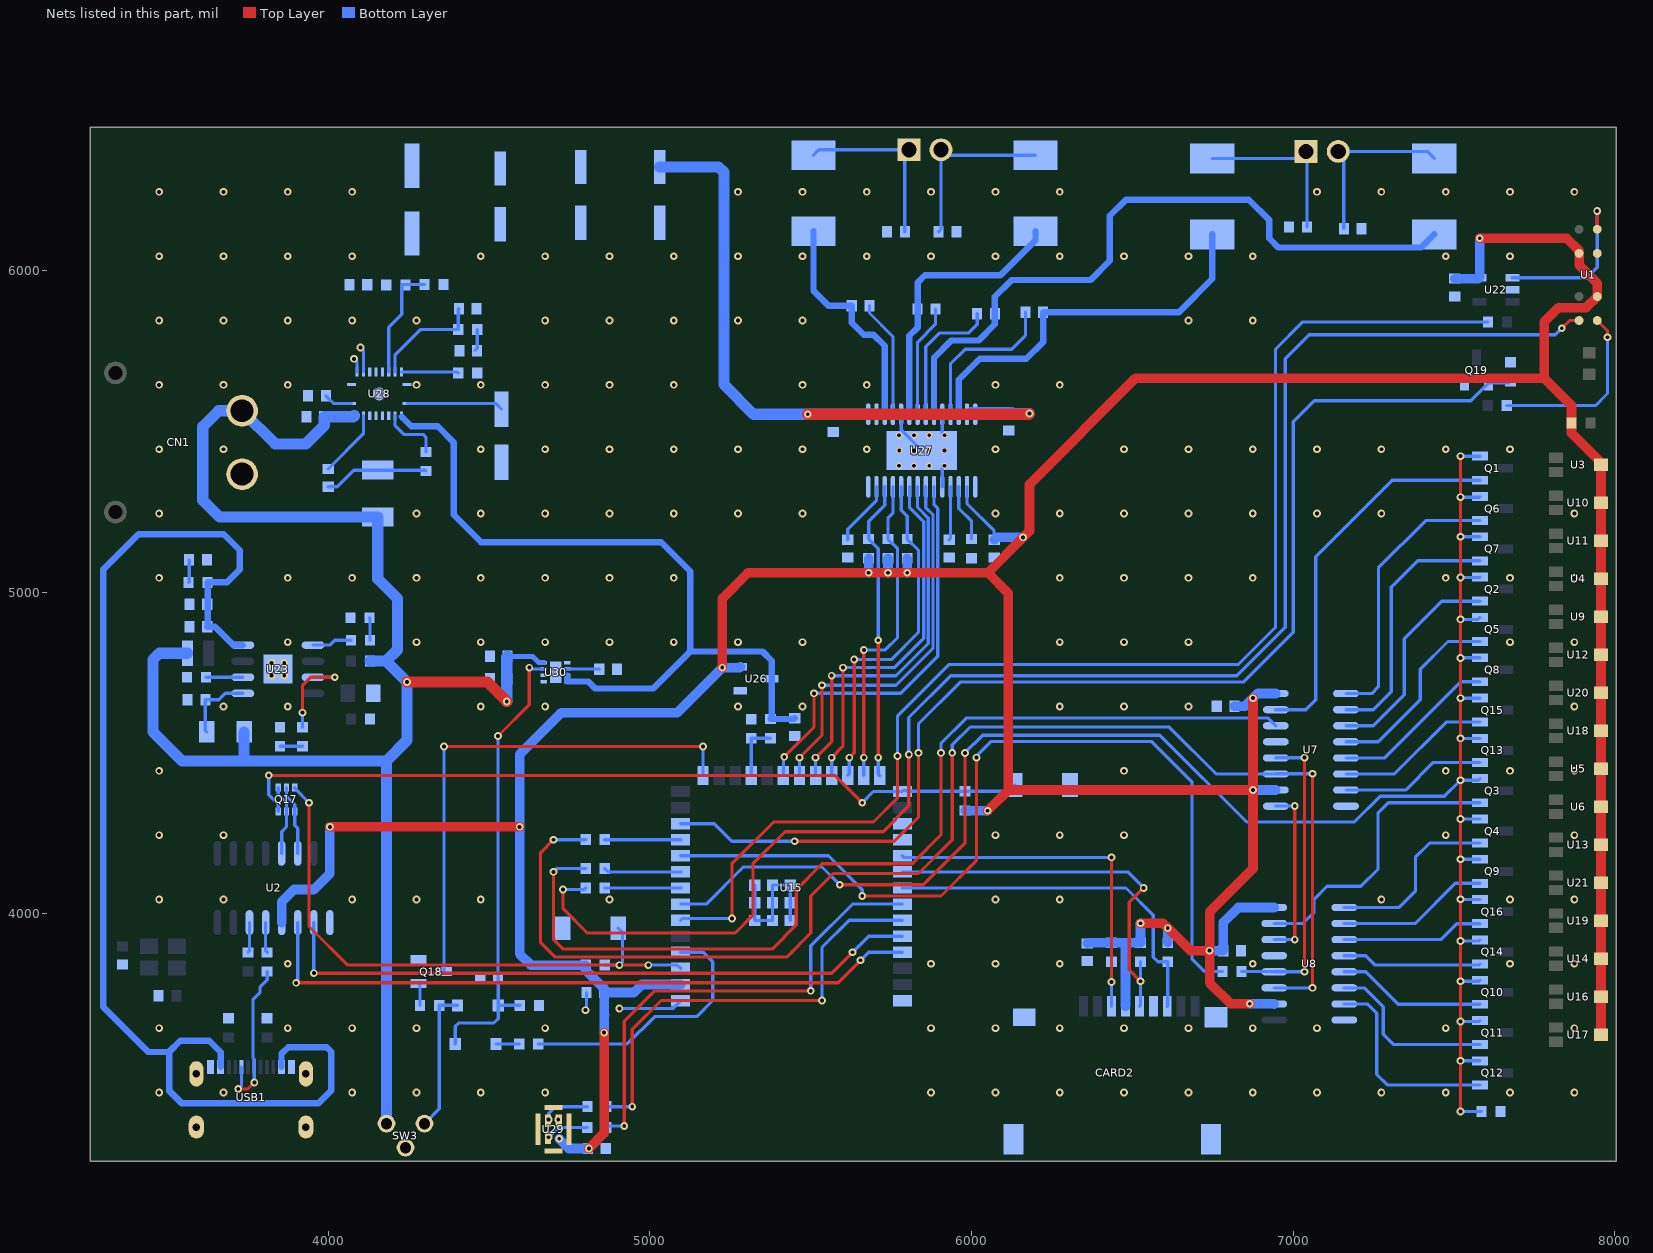
[diagram p0: the nets of this part, all layers, seen from the top]
# Altium PCB MISC75432.pcbdoc (part 2 of 2)
Units mil, origin at the board's own origin, x right, y up, seen from the top; angles counter-clockwise.
Board outline 4745 x 3215 mil, 2 copper layers (Top Layer, Bottom Layer), stack 62.206 mil thick; 150 components, 141 nets, 533 pads, 333 vias.

## Via types
v1: diameter 24.02, hole 12, Top Layer to Bottom Layer, 317 vias
v2: diameter 19.69, hole 11.8, Top Layer to Bottom Layer, 12 vias
v3: diameter 24, hole 12, Top Layer to Bottom Layer, 4 vias

## Nets (pads, with @x,y where several pads share a name; then routed paths per layer and width w, separated by ;. In a path a pad name is that pad's centre, name@x,y a point inside that pad or via, vN(x,y) a via of type N, cw(c..) or ccw(c..) an arc to the next point about the centre after c; other vN are vias at no path point) (continued)
$2N126: R16.1 U23.6 | length 114.7
  Bottom Layer w10: R16.1@3619.66,4735 U23.6@3734.37,4735
$2N139: C10.1 R19.2 | length 70.9
  Bottom Layer w10: R19.2@3565.34,5030 3567.44,5032.1 C10.1@3567.44,5100
$2N141: C9.2 R20.1 U23.5 | length 226.7
  Bottom Layer w10: R20.1@3621.78,4565 3617.68,4569.1 C9.2@3617.68,4665 3660,4665 3680,4685 U23.5@3734.37,4685
$2N142: LED2.2 R21.1 | length 70.1
  Bottom Layer w10: LED2.2@3849.99,4520.51 3919.83,4520.51 R21.1@3920,4520.34
$2N143: R21.2 U23.3 | length 308
  Top Layer w10: v1(3920,4625) 3920,4710 3945,4735 v1(4020,4735)
  Bottom Layer w10: R21.2@3920,4579.66 v1(3920,4625) ; U23.3@3952.67,4735 v1(4020,4735)
$2N144: R17.2 U23.1 | length 123.9
  Bottom Layer w10: U23.1@3952.67,4835 4005,4835 4020,4850 R17.2@4070.34,4850
$2N145: LED1.2 R17.1 | length 70.5
  Bottom Layer w10: LED1.2@4128.46,4919.98 4129.66,4918.79 R17.1@4129.66,4850
$2N168: D2.1 R26.2 | length 71.9
  Bottom Layer w10: D2.1@4521.57,3595.01 R26.2@4593.52,3595.01
$2N172: Q18.1 R27.1 | length 69.6
  Bottom Layer w10: Q18.1@4280.63,3782.6 4285.34,3777.89 R27.1@4285.34,3715
$2N183: C17.2 U28.1 | length 301.3
  Bottom Layer w10: U28.1@4244.44,5586.46 4520.62,5586.46 C17.2@4538.41,5568.66
$2N185: C18.2 L1.1 R30.2 U28.4 U28.5 U28.6 U28.7 | length 325.7
  Bottom Layer w10: C18.2@4000,5327.44 4027.32,5327.44 4078.69,5378.82 L1.1@4153.41,5378.82 4300.92,5378.82 R30.2@4303.41,5376.33
$2N186: R30.1 U28.3 | length 187.2
  Bottom Layer w10: U28.3@4207.55,5547.99 4207.55,5517.45 4235,5490 4295,5490 4303.41,5481.59 R30.1@4303.41,5435.65
$2N187: C18.1 U28.8 | length 210.6
  Bottom Layer w10: C18.1@4000,5382.56 4109.12,5491.68 U28.8@4109.12,5547.99
$2N197: R33.2 U28.19 | length 177.8
  Bottom Layer w10: U28.19@4227.23,5683.99 4400.75,5683.99 R33.2@4403.75,5680.99
$2N200: C20.1 R34.2 | length 68
  Bottom Layer w10: C20.1@4455.85,5750.99 4463.07,5758.21 R34.2@4463.07,5815.99
$2N209: R35.2 U27.3 | length 179
  Bottom Layer w10: U27.3@5960.16,5327.18 5960.16,5259.84 6000,5220 R35.2@6000,5164.66
$2N210: C27.1 U27.4 | length 166.5
  Bottom Layer w10: C27.1@5930,5162.56 5934.57,5167.13 U27.4@5934.57,5327.18
$2N219: C28.2 U27.13 | length 201.6
  Bottom Layer w10: C28.2@5615,5162.56 5615,5195 5704.25,5284.25 U27.13@5704.25,5327.18
$2N224: C33.1 U27.18 | length 367.4
  Bottom Layer w10: C33.1@5682.56,5890 5682.56,5867.44 5755.43,5794.57 U27.18@5755.43,5552.82
$2N227: C34.1 U27.21 | length 350.1
  Bottom Layer w10: U27.21@5832.2,5552.82 5832.2,5777.2 5887.56,5832.56 C34.1@5887.56,5880
$2N228: C35.1 U27.22 | length 431
  Bottom Layer w10: U27.22@5857.79,5552.82 5857.79,5762.79 5900,5805 5990,5805 6017.44,5832.44 C35.1@6017.44,5865
$2N231: C36.1 U27.25 | length 498.6
  Bottom Layer w10: U27.25@5934.57,5552.82 5934.57,5709.57 5980,5755 6125,5755 6167.44,5797.44 C36.1@6167.44,5870
$2N241: U15.29
$2N242: U15.30
$2N254: C38.1 CN3.1 L4.2 | length 563.5
  Bottom Layer w10: L4.2@5508.6,6358.11 5525.49,6375 CN3.1@5805,6374.99 5792.56,6362.56 C38.1@5792.56,6120
$2N255: C39.2 CN3.2 L5.2 | length 558.7
  Bottom Layer w10: C39.2@5897.44,6120 5905,6127.56 CN3.2@5905,6374.99 5921.89,6358.11 L5.2@6198.6,6358.11
$2N256: C30.1 CN2.1 L2.2 | length 536.5
  Bottom Layer w10: L2.2@6748.6,6348.11 7018.11,6348.11 CN2.1@7040,6369.99 7042.56,6367.44 C30.1@7042.56,6135
$2N257: C37.2 CN2.2 L3.2 | length 554.9
  Bottom Layer w10: C37.2@7157.44,6130 7157.44,6352.56 CN2.2@7140,6369.99 7416.71,6370 L3.2@7438.6,6348.11
$2N275: R39.2 U29.3 | length 149.3
  Bottom Layer w10: v1(4685,3360) 4685,3380 4705,3400 R39.2@4806.02,3400
$2N276: R40.2 U29.4 | length 132.6
  Bottom Layer w10: v1(4685,3305) 4715.34,3335.34 R40.2@4805,3335.34
$2N296: R11.2 U15.8 | length 235.9
  Bottom Layer w10: R11.2@4859.66,4080 5095.31,4080 U15.8@5095.51,4079.8
$2N298: R8.1 U15.9 | length 240.1
  Bottom Layer w10: R8.1@4859.66,4140 4869.85,4129.81 U15.9@5095.51,4129.81
$2N300: R9.1 U15.10 | length 2755.8
  Top Layer w10: v1(5660,4055) 5905,4055 6015,4165 v1(6015,4485)
  Bottom Layer w10: U15.10@5095.51,4179.81 5555.19,4179.81 5660,4075 v1(5660,4055) ; v1(6015,4485) 6015,4490 6060,4535 6560,4535 6685,4410 6685,3860 6725,3820 R9.1@6780.34,3820
$2N303: R10.2 U15.11 | length 235.9
  Bottom Layer w10: R10.2@4859.66,4230 4859.85,4229.81 U15.11@5095.51,4229.81
$2N304: D1.1 R27.2 SW3.2 | length 443.4
  Bottom Layer w10: SW3.2@4299.05,3347.4 4344.66,3393.01 R27.2@4344.66,3715 D1.1@4401.61,3715
$2N306: C22.1 U28.10 | length 89.6
  Bottom Layer w10: C22.1@3992.56,5610 4016.1,5586.46 U28.10@4072.39,5586.46
+12V: C19.1 C23.1 C24.1 C25.1 C29.1 C31.2 C32.2 R32.2 U27.15 U27.16 U27.27 U27.28 U28.14 U28.15 U28.16 | length 2234
  Top Layer w35: v1(5490.71,5552.56) 6177.56,5552.56 v1(6180,5555)
  Bottom Layer w35: C25.1@5030,6321.61 5213.39,6321.61 5230,6305 5230,5645 5322.44,5552.56 v1(5490.71,5552.56) C32.2@5570,5552.56 5694.24,5552.56 5694.51,5552.82 ; 5995.49,5552.82 6000.23,5557.56 C31.2@6115,5557.56 ; C31.2@6127.56,5555 v1(6180,5555)
AGND: C1.2 C2.2 C3.2 C4.1 C5.1 C6.2 C7.2 C8.1 C9.1 C10.2 C11.1 C12.2 C13.1 C14.1 C15.2 C16.2 C17.1 C19.2 C20.2 C21.2 C22.2 C23.2 C24.2 C25.2 C26.2 C27.2 C28.1 C29.2 C30.2 C31.1 C32.1 C37.1 C38.2 C39.1 C40.2 C41.2 CARD2.6 CARD2.10 CARD2.11 CARD2.12 CARD2.13 CN1.1 LED1.1 LED2.1 Q18.2 Q19.2 R1.2 R4.1 R7.1 R15.1 R16.2 R18.1 R25.2 R29.1 R31.1 R33.1 R35.1 R42.2 SW1.1 SW2.2 SW3.3 U1.3 U2.1 U7.8 U7.13 U8.8 U8.13 U15.1 U15.40 U15.41 U22.2 U23.9 U26.1 U27.1 U27.5 U27.14 U27.19 U27.24 U27.29 U28.11 U28.12 U28.13 U28.20 U28.21 U29.2 U29.5 U29.6 U29.7 U29.8 U30.5 U30.9 USB1.1 USB1.12 USB1.13 USB1.14 | length 1098.7
  Bottom Layer w10: v1(4080,5725) 4089.44,5715.56 U28.12@4089.44,5683.99 ; v1(4100,5760) 4109.12,5750.88 U28.13@4109.12,5683.99 ; v1(4800,3700) 4802.44,3702.44 C13.1@4802.44,3755 ; v1(4905,3705) 5070.7,3705 U15.1@5095.51,3729.8 ; U15.41@5325.82,4088.86 U15.41@5325.82,4033.74 U15.41@5325.82,3978.62 U15.41@5380.94,3978.62 U15.41@5380.94,4033.74 U15.41@5380.94,4088.86 U15.41@5436.06,4088.86 U15.41@5436.06,4033.74 U15.41@5436.06,3978.62 ; U27.19@5781.02,5552.82 5781.02,5503.98 U27.29@5845,5439.99 ; U27.5@5908.98,5327.18 5908.98,5385.86 v2(5915.87,5392.76) ; U27.24@5908.98,5552.82 5908.98,5494.14 v2(5915.87,5487.24)
  other v1: 4715,3360 3474.1,3444.1 3674.1,3444.1 4074.1,3444.1 4274.1,3444.1 4474.1,3444.1 4674.1,3444.1 5874.1,3444.1 6074.1,3444.1 6274.1,3444.1 6474.1,3444.1 6674.1,3444.1 6874.1,3444.1 7074.1,3444.1 7274.1,3444.1 7474.1,3444.1 7674.1,3444.1 7874.1,3444.1 3474.1,3644.1 3874.1,3644.1 4074.1,3644.1 4274.1,3644.1 4674.1,3644.1 5874.1,3644.1 6074.1,3644.1 6274.1,3644.1 6474.1,3644.1 6674.1,3644.1 6874.1,3644.1 7074.1,3644.1 7474.1,3644.1 7874.1,3644.1 3874.1,3844.1 5874.1,3844.1 6074.1,3844.1 6274.1,3844.1 6874.1,3844.1 7674.1,3844.1 7874.1,3844.1 3474.1,4044.1 3674.1,4044.1 4074.1,4044.1 4274.1,4044.1 4474.1,4044.1 4874.1,4044.1 6074.1,4044.1 6274.1,4044.1 7274.1,4044.1 7674.1,4044.1 7874.1,4044.1 3474.1,4244.1 3674.1,4244.1 6074.1,4244.1 6274.1,4244.1 6474.1,4244.1 7474.1,4244.1 7874.1,4244.1 3474.1,4444.1 6474.1,4444.1 7474.1,4444.1 7674.1,4444.1 7874.1,4444.1 3674.1,4644.1 3874.1,4644.1 4474.1,4644.1 4674.1,4644.1 5274.1,4644.1 5474.1,4644.1 6274.1,4644.1 6474.1,4644.1 6674.1,4644.1 7874.1,4644.1 3874.1,4844.1 4274.1,4844.1 4474.1,4844.1 4674.1,4844.1 4874.1,4844.1 5074.1,4844.1 5274.1,4844.1 5474.1,4844.1 6274.1,4844.1 6474.1,4844.1 6674.1,4844.1 7674.1,4844.1 7874.1,4844.1 3474.1,5044.1 3874.1,5044.1 4074.1,5044.1 4274.1,5044.1 4474.1,5044.1 4674.1,5044.1 4874.1,5044.1 5074.1,5044.1 6274.1,5044.1 6474.1,5044.1 6674.1,5044.1 6874.1,5044.1 7474.1,5044.1 7674.1,5044.1 7874.1,5044.1 3474.1,5244.1 4274.1,5244.1 4474.1,5244.1 4674.1,5244.1 4874.1,5244.1 5074.1,5244.1 5274.1,5244.1 5474.1,5244.1 6074.1,5244.1 6274.1,5244.1 6474.1,5244.1 6674.1,5244.1 6874.1,5244.1 7074.1,5244.1 7274.1,5244.1 7874.1,5244.1 3474.1,5444.1 3674.1,5444.1 4474.1,5444.1 4674.1,5444.1 4874.1,5444.1 5074.1,5444.1 5274.1,5444.1 5474.1,5444.1 5674.1,5444.1 6074.1,5444.1 6474.1,5444.1 6674.1,5444.1 6874.1,5444.1 7074.1,5444.1 7274.1,5444.1 7474.1,5444.1 7674.1,5444.1 3474.1,5644.1 3674.1,5644.1 3874.1,5644.1 4274.1,5644.1 4474.1,5644.1 4674.1,5644.1 4874.1,5644.1 5074.1,5644.1 5474.1,5644.1 5674.1,5644.1 6074.1,5644.1 6274.1,5644.1 3474.1,5844.1 3674.1,5844.1 3874.1,5844.1 4074.1,5844.1 4274.1,5844.1 4674.1,5844.1 4874.1,5844.1 5074.1,5844.1 5274.1,5844.1 5474.1,5844.1 6674.1,5844.1 6874.1,5844.1 3474.1,6044.1 3674.1,6044.1 3874.1,6044.1 4074.1,6044.1 4474.1,6044.1 4674.1,6044.1 4874.1,6044.1 5074.1,6044.1 5274.1,6044.1 5474.1,6044.1 5674.1,6044.1 5874.1,6044.1 6074.1,6044.1 6274.1,6044.1 6474.1,6044.1 6674.1,6044.1 6874.1,6044.1 7474.1,6044.1 7674.1,6044.1 3474.1,6244.1 3674.1,6244.1 3874.1,6244.1 4074.1,6244.1 5274.1,6244.1 5474.1,6244.1 5674.1,6244.1 5874.1,6244.1 6074.1,6244.1 6274.1,6244.1 7074.1,6244.1 7274.1,6244.1 7474.1,6244.1 7674.1,6244.1 7874.1,6244.1
  other v2: 5774.13,5392.76 5821.38,5392.76 5868.62,5392.76 5775,5439.99 5821.38,5439.99 5868.62,5439.99 5915.87,5439.99 5774.13,5487.24 5821.38,5487.24 5868.62,5487.24
  other v3: 3823.84,4740.31 3863.21,4740.31 3823.84,4779.68 3863.21,4779.68
AMP_PDN: R36.2 U15.26 U27.12 | length 933.3
  Top Layer w10: v1(5710,4485) v1(5710,4850)
  Bottom Layer w10: v1(5710,4485) 5710,4434.02 U15.26@5715,4429.02 ; v1(5710,4850) 5710,5134.66 R36.2@5680,5164.66 5680,5220 5729.84,5269.84 U27.12@5729.84,5327.18
AMP_SCL: R38.2 U15.25 U27.11 | length 998.2
  Top Layer w10: v1(5665,4485) v1(5665,4820)
  Bottom Layer w10: U15.25@5665,4430.19 v1(5665,4485) ; v1(5665,4820) 5731.42,4820 5770,4858.58 5770,5134.66 R38.2@5740,5164.66 5740,5230 5755.43,5245.43 U27.11@5755.43,5327.18
AMP_SDA: R37.2 U15.24 U27.10 | length 1077.8
  Top Layer w10: v1(5620,4485) 5635,4500 v1(5635,4790)
  Bottom Layer w10: U15.24@5615,4430.19 5620,4435.19 v1(5620,4485) ; v1(5635,4790) 5750,4790 5835,4875 5835,5129.66 R37.2@5800,5164.66 5800,5235 5781.02,5253.98 U27.10@5781.02,5327.18
BAT_MONITOR: R28.1 R29.2 U15.18 | length 174.9
  Bottom Layer w10: U15.18@5315,4430.19 R29.2@5315,4545.34 5374.32,4545.34 R28.1@5374.66,4545.68
CH340G_RXD: U2.3 U15.37 | length 2113.1
  Top Layer w10: v1(3900,3785) 5585,3785 v1(5655,3855)
  Bottom Layer w10: v1(3900,3785) 3905,3790 U2.3@3905,3972.3 ; v1(5655,3855) 5679.81,3879.8 U15.37@5784.49,3879.8
CH340G_TXD: U2.2 U15.36 | length 2034.3
  Top Layer w10: v1(3955,3815) 5565,3815 v1(5630,3880)
  Bottom Layer w10: v1(3955,3815) U2.2@3955,3972.3 ; v1(5630,3880) 5679.81,3929.8 U15.36@5784.49,3929.8
COMP: C21.1 R34.1 U28.18 | length 348.1
  Bottom Layer w10: U28.18@4207.55,5683.99 4207.55,5737.55 4285.99,5815.99 R34.1@4403.75,5815.99 4403.75,5878.89 C21.1@4405.85,5880.99
CT: C41.1 U30.6 | length 99.8
  Bottom Layer w10: U30.6@4743.1,4761.05 4841.39,4761.05 C41.1@4842.44,4760
D+: R6.1 U2.5 | length 94.7
  Bottom Layer w10: U2.5@3805,3972.3 3805,3884.66 R6.1@3810,3879.66
D-: R5.1 U2.6 | length 94.7
  Bottom Layer w10: R5.1@3750,3879.66 3755,3884.66 U2.6@3755,3972.3
DP1: R6.2 USB1.6 USB1.8 | length 496.4
  Top Layer w10: v1(3720,3455) 3750,3455 v1(3770,3475)
  Bottom Layer w10: v1(3720,3455) 3730,3465 3730,3523.03 USB1.8@3730.47,3523.51 ; v1(3770,3475) 3769.84,3475.16 USB1.6@3769.84,3523.51 3769.84,3546.91 3766,3550.75 3766,3733.84 3788,3755.84 3788,3772.46 3810,3794.46 R6.2@3810,3820.34
DTR: Q17.2 Q17.4 U2.13 | length 221.5
  Bottom Layer w10: Q17.4@3844.41,4392.4 3844.41,4370.59 3870,4345 Q17.2@3870,4317.6 3870,4270 3855,4255 U2.13@3855,4187.7
FB: R31.2 R32.1 U28.17 | length 359.3
  Bottom Layer w10: U28.17@4187.86,5683.99 4187.86,5822.86 4228.07,5863.07 4228.07,5955.99 R31.2@4298.75,5955.99
I2S_LRCK: U15.20 U27.6 | length 1258.8
  Top Layer w10: v1(5417.5,4487.5) 5510,4580 v1(5510,4685)
  Bottom Layer w10: U15.20@5415,4430.19 5415,4485 v1(5417.5,4487.5) ; v1(5510,4685) 5780,4685 5895,4800 5895,5260 5883.39,5271.61 U27.6@5883.39,5327.18
I2S_SCLK: U15.21 U27.7 | length 1212.8
  Top Layer w10: v1(5465,4485) 5535,4555 v1(5535,4710)
  Bottom Layer w10: U15.21@5465,4430.19 v1(5465,4485) ; v1(5535,4710) 5765,4710 5880,4825 5880,5240 5857.79,5262.21 U27.7@5857.79,5327.18
I2S_SDIN: U15.22 U27.8 | length 1172.7
  Top Layer w10: v1(5515,4485) 5565,4535 v1(5565,4740)
  Bottom Layer w10: U15.22@5515,4430.19 v1(5515,4485) ; v1(5565,4740) 5765,4740 5865,4840 5865,5230 5832.2,5262.8 U27.8@5832.2,5327.18
I2S_SDOUT: U15.23 U27.9 | length 1127.5
  Top Layer w10: v1(5565,4485) 5600,4520 v1(5600,4765)
  Bottom Layer w10: U15.23@5565,4430.19 v1(5565,4485) ; v1(5600,4765) 5760,4765 5850.98,4855.98 5850.98,5219.02 5806.61,5263.39 U27.9@5806.61,5327.18
IO0: Q17.3 R3.1 SW2.1 U15.27 | length 2503.5
  Top Layer w10: v1(3815,4430) 5575,4430 v1(5660,4345)
  Bottom Layer w10: v1(3815,4430) 3815,4370 3844.41,4340.59 Q17.3@3844.41,4317.6 ; v1(5660,4345) 5694.81,4379.81 U15.27@5784.49,4379.81 5787.34,4382.66 5797.34,4382.66 5799.66,4380.34 R3.1@5980,4380.34 6114.32,4380.34 SW2.1@6133.98,4400
LED_PWM: Q19.1 R42.1 U15.12 | length 3748.2
  Top Layer w10: v1(5450,4225) 5760,4225 5835,4300 v1(5835,4500)
  Bottom Layer w10: U15.12@5095.51,4279.81 5200.19,4279.81 5255,4225 v1(5450,4225) ; v1(5835,4500) 5835,4590 5965,4720 6845,4720 7000,4875 7000,5530 7065,5595 7551.77,5595 Q19.1@7607.4,5650.63 7670.29,5650.63 R42.1@7675,5655.34
OUT_A+: C36.2 L2.1 U27.26 | length 1218
  Bottom Layer w19.68: U27.26@5960.16,5552.82 5960.16,5660.16 6025,5725 6170,5725 6222.56,5777.56 C36.2@6222.56,5870 6645,5870 6748.6,5973.6 L2.1@6748.6,6111.89
OUT_A-: C35.2 L3.1 U27.23 | length 2178
  Bottom Layer w19.68: U27.23@5883.39,5552.82 5883.39,5728.39 5937.17,5782.17 6022.17,5782.17 6072.56,5832.56 C35.2@6072.56,5865 6072.56,5917.56 6125,5970 6370,5970 6430,6030 6430,6170 6480,6220 6861.61,6220 6925,6156.61 6925,6100 6953.92,6071.08 7397.79,6071.08 L3.1@7438.6,6111.89
OUT_B+: C33.2 L4.1 U27.17 | length 720.7
  Bottom Layer w19.68: L4.1@5508.6,6121.89 5508.6,5936.4 5555,5890 C33.2@5627.44,5890 5627.44,5837.56 5665,5800 5695,5800 5729.84,5765.16 U27.17@5729.84,5552.82
OUT_B-: C34.2 L5.1 U27.20 | length 869.1
  Bottom Layer w19.68: U27.20@5806.61,5552.82 5806.61,5796.61 5832.44,5822.44 C34.2@5832.44,5880 5832.44,5962.44 5855,5985 6090,5985 6198.6,6093.6 L5.1@6198.6,6121.89
PD_GATE_1: Q1.1 U7.15 | length 1190.8
  Bottom Layer w10: U7.15@6945.98,4634.33 7039.33,4634.33 7070,4665 7070,5110 7307.6,5347.6 Q1.1@7580.63,5347.6
PD_GATE_2: Q6.1 U7.1 | length 856.2
  Bottom Layer w10: U7.1@7164.02,4684.33 7244.33,4684.33 7265,4705 7265,5075 7412.27,5222.27 Q6.1@7580.63,5222.27
PD_GATE_3: Q7.1 U7.2 | length 798.6
  Bottom Layer w10: U7.2@7164.02,4634.33 7249.33,4634.33 7305,4690 7305,5015 7386.93,5096.93 Q7.1@7580.63,5096.93
PD_GATE_4: Q2.1 U7.3 | length 679.5
  Bottom Layer w10: U7.3@7164.02,4584.33 7249.33,4584.33 7345,4680 7345,4855 7461.6,4971.6 Q2.1@7580.63,4971.6
PD_GATE_5: Q5.1 U7.4 | length 601.5
  Bottom Layer w10: U7.4@7164.02,4534.33 7264.33,4534.33 7395,4665 7395,4760 7481.27,4846.27 Q5.1@7580.63,4846.27
PD_GATE_6: Q8.1 U7.5 | length 514.6
  Bottom Layer w10: U7.5@7164.02,4484.33 7284.33,4484.33 7520.93,4720.93 Q8.1@7580.63,4720.93
PD_GATE_7: Q15.1 U7.6 | length 483.4
  Bottom Layer w10: U7.6@7164.02,4434.33 7314.33,4434.33 7475.6,4595.6 Q15.1@7580.63,4595.6
PD_GATE_8: Q13.1 U7.7 | length 452.2
  Bottom Layer w10: U7.7@7164.02,4384.33 7349.33,4384.33 7435.27,4470.27 Q13.1@7580.63,4470.27
PD_GATE_9: Q3.1 U8.15 | length 921.2
  Bottom Layer w10: U8.15@6940.98,3969.33 7029.33,3969.33 7065,4005 7065,4045 7105,4085 7210,4085 7263.86,4138.86 7263.86,4313.86 7294.93,4344.93 Q3.1@7580.63,4344.93
PD_GATE_10: Q4.1 U8.1 | length 566.1
  Bottom Layer w10: U8.1@7159.02,4019.33 7329.33,4019.33 7380,4070 7380,4175 7424.6,4219.6 Q4.1@7580.63,4219.6
PD_GATE_11: Q9.1 U8.2 | length 473.4
  Bottom Layer w10: U8.2@7159.02,3969.33 7379.33,3969.33 7504.27,4094.27 Q9.1@7580.63,4094.27
PD_GATE_12: Q16.1 U8.3 | length 442.2
  Bottom Layer w10: U8.3@7159.02,3919.33 7459.33,3919.33 7508.93,3968.93 Q16.1@7580.63,3968.93
PD_GATE_13: Q14.1 U8.4 | length 435.3
  Bottom Layer w10: U8.4@7159.02,3869.33 7225.67,3869.33 7255,3840 7577.03,3840 Q14.1@7580.63,3843.6
PD_GATE_14: Q10.1 U8.5 | length 463.5
  Bottom Layer w10: U8.5@7159.02,3819.33 7225.67,3819.33 7326.73,3718.27 Q10.1@7580.63,3718.27
PD_GATE_15: Q11.1 U8.6 | length 544.5
  Bottom Layer w10: U8.6@7159.02,3769.33 7220.67,3769.33 7280,3710 7280,3625 7312.07,3592.93 Q11.1@7580.63,3592.93
PD_GATE_16: Q12.1 U8.7 | length 637.2
  Bottom Layer w10: U8.7@7159.02,3719.33 7230.67,3719.33 7260,3690 7260,3500 7292.4,3467.6 Q12.1@7580.63,3467.6
PD_OUT: Q1.2 Q2.2 Q3.2 Q4.2 Q5.2 Q6.2 Q7.2 Q8.2 Q9.2 Q10.2 Q11.2 Q12.2 Q13.2 Q14.2 Q15.2 Q16.2 R1.1 U15.7 | length 6101.1
  Top Layer w10: v1(5590,4090) 5850,4090 5979.24,4219.24 v1(5979.24,4499.86) ; v1(7520,3385) v1(7520,3542.4) v1(7520,3665) v1(7520,3790) v1(7520,3915) v1(7520,4045) v1(7520,4169.07) v1(7520,4294.4) v1(7520,4415) v1(7520,4545) v1(7520,4670) v1(7520,4795) v1(7520,4915) v1(7520,5045) v1(7520,5171.73) v1(7520,5295) v1(7520,5422.4)
  Bottom Layer w10: U15.7@5095.51,4029.8 5174.81,4029.8 5290,4145 5535,4145 v1(5590,4090) ; v1(5979.24,4499.86) 6034.38,4555 6585,4555 6855,4285 7190,4285 7270,4365 7470,4365 v1(7520,4415) 7575.9,4415 Q3.2@7580.63,4419.73 ; v1(7520,3385) R1.1@7585.34,3385 ; v1(7520,3542.4) Q12.2@7580.63,3542.4 ; v1(7520,3665) 7577.9,3665 Q11.2@7580.63,3667.73 ; v1(7520,3790) 7577.56,3790 Q10.2@7580.63,3793.07 ; v1(7520,3915) 7577.23,3915 Q14.2@7580.63,3918.4 ; v1(7520,4045) 7521.27,4043.73 Q16.2@7580.63,4043.73 ; v1(7520,4169.07) Q9.2@7580.63,4169.07 ; v1(7520,4294.4) Q4.2@7580.63,4294.4 ; v1(7520,4545) Q13.2@7580.56,4545 ; v1(7520,4670) 7580.23,4670 Q15.2@7580.63,4670.4 ; v1(7520,4795) 7520.73,4795.73 Q8.2@7580.63,4795.73 ; v1(7520,4915) 7574.56,4915 Q5.2@7580.63,4921.07 ; v1(7520,5045) 7579.23,5045 Q2.2@7580.63,5046.4 ; v1(7520,5171.73) Q7.2@7580.63,5171.73 ; v1(7520,5295) 7578.56,5295 Q6.2@7580.63,5297.07 ; v1(7520,5422.4) Q1.2@7580.63,5422.4
PDM_CLK: R39.1 U15.35 | length 1396.6
  Top Layer w10: v1(4945,3400) 4945,3640 5035,3730 v1(5535,3730)
  Bottom Layer w10: R39.1@4865.34,3400 v1(4945,3400) ; v1(5535,3730) 5535,3895 5619.81,3979.8 U15.35@5784.49,3979.8
PDM_DATA: R40.1 U15.34 | length 1480.2
  Top Layer w10: v1(4920,3340) 4920,3665 5015,3760 v1(5500,3760)
  Bottom Layer w10: R40.1@4864.32,3335.34 4868.98,3340 v1(4920,3340) ; v1(5500,3760) 5500,3900 5629.81,4029.8 U15.34@5784.49,4029.8
PWR_EN: C12.1 D1.2 D2.2 R25.1 U30.3 | length 1444.1
  Top Layer w10: v1(4527.56,4552.44) 4625,4649.88 v1(4625,4765)
  Bottom Layer w10: D2.2@4394.79,3595.01 4394.79,3649.79 4405,3660 4515,3660 4528.39,3673.39 D1.2@4528.39,3715 ; v1(4527.56,4552.44) C12.1@4527.56,3800 4528.39,3799.17 D1.2@4528.39,3715 ; R25.1@4595.34,3715 D1.2@4528.39,3715 ; v1(4625,4765) 4628.95,4761.05 U30.3@4670.06,4761.05
PWR_HOLD: R26.1 U15.4 | length 829.9
  Bottom Layer w10: R26.1@4652.84,3595.01 4930.01,3595.01 5015,3680 5145,3680 5195,3730 5195,3850 5165.19,3879.8 U15.4@5095.51,3879.8
PWR_KEY_SENSE: Q18.3 U15.15 | length 1595.4
  Top Layer w10: v1(4359.37,4520) v1(5165,4520)
  Bottom Layer w10: Q18.3@4359.37,3820 v1(4359.37,4520) ; U15.15@5165,4430.19 v1(5165,4520)
RAW_VIDEO: U1.4 U22.1 | length 509.9
  Top Layer w10: v1(7945,6185) 7945,6128.13 U1.4@7945.5,6127.63
  Bottom Layer w10: U22.1@7681.19,5977.4 7912.4,5977.4 7945,6010 v1(7945,6185)
RESET: Q17.6 R13.2 SW1.2 U15.3 | length 1830.5
  Top Layer w10: v1(3940,4345) 3940,3960 4060,3840 v1(4905,3840) v1(4995,3840)
  Bottom Layer w10: Q17.6@3895.59,4392.4 3895.59,4389.41 v1(3940,4345) ; R13.2@4859.66,3840 v1(4905,3840) 4915,3850 4915,3941.02 SW1.2@4901.02,3955 ; v1(4995,3840) 5085.31,3840 U15.3@5095.51,3829.8
RTS: Q17.1 Q17.5 U2.14 | length 219.2
  Bottom Layer w10: Q17.5@3870,4392.4 3870,4365 3895.59,4339.41 Q17.1@3895.59,4317.6 3895.59,4274.41 3905,4265 U2.14@3905,4187.7
S13131_CLK: R12.1 U1.1 | length 568.7
  Top Layer w10: U1.1@7945.5,5844.17 7977.14,5812.52 v1(7977.14,5792.14)
  Bottom Layer w10: R12.1@7663.98,5580 7940,5580 7977.14,5617.14 v1(7977.14,5792.14)
S13131_OUT: R2.2 U15.6 | length 4036
  Top Layer w10: v1(5255,3985) 5255,4155 5385,4285 5695,4285 5770,4360 v1(5770,4490)
  Bottom Layer w10: U15.6@5095.51,3979.8 5100.7,3985 v1(5255,3985) ; v1(5770,4490) 5770,4615 5930,4775 6830,4775 6945,4890 6945,5755 7030,5840 R2.2@7605.34,5840
S13131_ST: R11.1 U1.8 | length 4855
  Top Layer w10: v1(4730,4075) 4730,4015 4805,3940 5265,3940 5320,3995 5320,4155 5420,4255 5725,4255 5805,4335 v1(5805,4495) ; v1(7835,5820) 7859.17,5844.17 U1.8@7888.81,5844.17
  Bottom Layer w10: v1(4730,4075) 4795.34,4075 R11.1@4800.34,4080 ; v1(5805,4495) 5805,4610 5935,4740 6825,4740 6975,4890 6975,5725 7050,5800 7815,5800 v1(7835,5820)
SD_CLK: CARD2.5 R23.2 U15.32 | length 1234.2
  Top Layer w10: v1(6525,3790) 6490,3825 6490,4035 v1(6535,4080)
  Bottom Layer w10: U15.32@5784.49,4129.81 6485.19,4129.81 v1(6535,4080) ; CARD2.5@6521.77,3711.75 6525,3714.98 v1(6525,3790) R23.2@6525,3850.34
SD_CMD: CARD2.3 R22.2 U15.31 | length 1178.3
  Top Layer w10: v1(6435,3787.84) v1(6435,4175)
  Bottom Layer w10: U15.31@5784.49,4179.81 5789.3,4175 v1(6435,4175) ; R22.2@6435,3850.34 v1(6435,3787.84) 6435,3711.91 CARD2.3@6435.16,3711.75
SD_DATA: CARD2.7 R24.2 U15.33 | length 1136
  Bottom Layer w10: U15.33@5784.49,4079.8 6480.19,4079.8 6565,3995 6565,3865 6579.66,3850.34 R24.2@6610,3850.34 6610,3713.36 CARD2.7@6608.39,3711.75
SER_OUT: U7.9 U8.14 | length 539
  Top Layer w10: v1(7005,3919.33) v1(7005,4335)
  Bottom Layer w10: U8.14@6940.98,3919.33 v1(7005,3919.33) ; U7.9@6945.98,4334.33 6946.65,4335 v1(7005,4335)
SR_CLK: R10.1 U7.11 U8.11 | length 4237.2
  Top Layer w10: v1(4700,4230) 4660,4190 4660,3910 4705,3865 5425,3865 5500,3940 5500,4055 5570,4125 5835,4125 5940,4230 v1(5940,4500) ; v1(7060,3769.33) v1(7060,4435)
  Bottom Layer w10: v1(4700,4230) R10.1@4800.34,4230 ; v1(5940,4500) 5940,4525 5995,4580 6615,4580 6760.67,4434.33 U7.11@6945.98,4434.33 6946.65,4435 v1(7060,4435) ; U8.11@6940.98,3769.33 v1(7060,3769.33)
SR_DATA: R8.2 U7.14 | length 3111.4
  Top Layer w10: v1(4700,4130) 4700,3920 4730,3890 5380,3890 5455,3965 5455,4075 5535,4155 5815,4155 5905,4245 v1(5905,4500)
  Bottom Layer w10: v1(4700,4130) 4710,4140 R8.2@4800.34,4140 ; v1(5905,4500) 5905,4530 5982.96,4607.96 6922.35,4607.96 U7.14@6945.98,4584.33
SR_LATCH: R9.2 U7.12 U8.12 | length 950.6
  Top Layer w10: v1(7035,3819.33) v1(7035,4485)
  Bottom Layer w10: R9.2@6839.66,3820 6940.31,3820 U8.12@6940.98,3819.33 v1(7035,3819.33) ; U7.12@6945.98,4484.33 6946.65,4485 v1(7035,4485)
VBAT: C8.2 C15.1 C16.1 CN1.2 L1.2 R14.1 R20.2 SW3.1 U24.2 U28.9 U30.1 U30.2 U30.4 | length 5200.9
  Top Layer w35: v1(4245,4720) 4495,4720 v1(4555,4660)
  Bottom Layer w15.75: C16.1@4557.44,4800 4635,4800 4654.26,4780.74 U30.4@4670.06,4780.74
  Bottom Layer w35: U24.2@3562.32,4810 3475,4810 3455,4790 3455,4565 3545,4475 3738.22,4475 ; R20.2@3738.22,4565 3738.22,4475 ; 4080.84,5547.99 4077.85,5545 C15.1@3987.56,5545 3987.56,5517.56 3930,5460 3835.28,5460 CN1.2@3731.85,5563.42 3658.43,5563.43 3610,5515 3610,5285 3661.84,5233.16 L1.2@4153.41,5233.16 4153.41,5041.59 4215,4980 4215,4820.68 4179.66,4785.34 ; R14.1@4129.66,4785.34 4179.66,4785.34 ; SW3.1@4180.94,3347.4 4180.94,4475 ; v1(4555,4660) 4555,4797.56 C16.1@4557.44,4800 ; 3738.22,4475 4180.94,4475 ; 4179.66,4785.34 v1(4245,4720) 4245,4539.06 4180.94,4475
VBUS: C6.1 C7.1 R19.1 U23.8 USB1.2 USB1.11 | length 3787.5
  Bottom Layer w20: USB1.11@3665.51,3523.51 3665.51,3569.49 3630,3605 3540,3605 3505,3570 ; U23.8@3734.37,4835 3705,4835 3647.5,4892.5 C6.1@3623.59,4892.5 3624.66,4893.57 R19.1@3624.66,5030 3685,5030 3725,5070 3725,5130 3675,5180 3410,5180 3300,5070 3300,3710 3440,3570 3505,3570 ; USB1.2@3854.49,3523.51 3854.49,3564.49 3875,3585 3995,3585 4009.14,3570.86 4009.14,3450 3969.14,3410 3545,3410 3505,3450 3505,3570
VCC: C1.1 C2.1 C3.1 C11.2 C13.2 C26.1 C40.1 CARD2.4 R3.2 R13.1 R22.1 R23.1 R24.1 R36.1 R37.1 R38.1 R41.1 U1.2 U1.6 U2.4 U2.16 U3.3 U4.3 U5.3 U6.3 U7.10 U7.16 U8.10 U8.16 U9.3 U10.3 U11.3 U12.3 U13.3 U14.3 U15.2 U16.3 U17.3 U18.3 U19.3 U20.3 U21.3 U22.5 U26.2 U27.2 U29.1 | length 14379.9
  Top Layer w30: v1(4005,4270) v1(4595,4270) ; v1(4810,3270) 4857.56,3317.56 v1(4857.56,3630) ; v1(5225,4765) 5225,4980 5305,5060 v1(5680,5060) v1(5740,5060) v1(5800,5060) 6050.4,5060 ; v1(6050,4320) 6114.33,4384.33 ; v1(6160,5170) v1@6160.4,5170 ; v1(6525,3970) 6595,3970 v1(6610,3955) 6680,3885 v1(6740,3885) ; v1(6865,3720) 6805,3720 6740,3785 v1(6740,3885) ; v1(6875,4670) v1(6875,4384.33) ; v1(7580,6100) 7850,6100 7888.81,6061.19 U1.6@7888.81,6052.83 7888.81,6016.19 7945.5,5959.5 U1.2@7945.5,5918.97 7910.74,5884.2 7824.2,5884.2 7780,5840 7780,5665 ; U17.3@7956.89,3623.7 U16.3@7956.89,3741.81 U14.3@7956.89,3859.92 U19.3@7956.89,3978.03 U21.3@7956.89,4096.14 U13.3@7956.89,4214.25 U6.3@7956.89,4332.36 U5.3@7956.89,4450.47 U18.3@7956.89,4568.58 U20.3@7956.89,4686.69 U12.3@7956.89,4804.8 U9.3@7956.89,4922.91 U4.3@7956.89,5041.02 U11.3@7956.89,5159.13 U10.3@7956.89,5277.24 U3.3@7956.89,5395.35 7956.89,5403.11 7865.34,5494.66 R41.1@7865.34,5525 7865.34,5579.66 7780,5665 ; 6050.4,5060 6114.33,4996.07 6114.33,4384.33 ; 6050.4,5060 v1@6160.4,5170 ; 6114.33,4384.33 v1(6875,4384.33) ; v1@6160.4,5170 6180,5189.6 6180,5335 6510,5665 7780,5665 ; v1(6740,3885) 6740,4005 6875,4140 v1(6875,4384.33)
  Bottom Layer w10: U27.2@5985.75,5327.18 5985.75,5274.25 6070,5190 C26.1@6070,5162.56
  Bottom Layer w30: U2.4@3855,3972.3 3855,4036.74 3893.26,4075 3955,4075 4005,4125 U2.16@4005,4187.7 v1(4005,4270) ; v1(4717.99,3300) 4747.99,3270 v1(4810,3270) ; v1(4857.56,3630) 4857.56,3687.44 ; 4860,3685 4857.56,3687.44 ; U15.2@5095.51,3779.8 4974.81,3779.8 4950,3755 C13.2@4857.56,3755 ; U26.2@5281.38,4767.4 5278.98,4765 v1(5225,4765) 5085,4625 4725,4625 4595,4495 v1(4595,4270) 4595,3875 4630,3840 R13.1@4800.34,3840 4800.34,3824.66 4857.56,3767.44 C13.2@4857.56,3755 ; v1(5680,5060) R36.1@5680,5105.34 ; v1(5740,5060) R38.1@5740,5105.34 ; v1(5800,5060) R37.1@5800,5105.34 ; R3.2@5980,4321.02 5981.02,4320 v1(6050,4320) ; C26.1@6070,5162.56 6077.44,5170 v1(6160,5170) ; C11.2@6360,3907.56 6362.1,3909.66 R22.1@6435,3909.66 6474.1,3909.66 ; CARD2.4@6478.47,3711.75 6478.47,3905.29 6474.1,3909.66 ; v1(6525,3970) R23.1@6525,3909.66 6474.1,3909.66 ; R24.1@6610,3909.66 v1(6610,3955) ; v1(6740,3885) C2.1@6782.44,3885 6782.44,3972.44 6829.33,4019.33 U8.16@6940.98,4019.33 ; C1.1@6817.56,4645 6850,4645 v1(6875,4670) 6889.33,4684.33 U7.16@6945.98,4684.33 ; v1(6865,3720) 6940.31,3720 U8.10@6940.98,3719.33 ; v1(6875,4384.33) U7.10@6945.98,4384.33 ; C3.1@7502.44,5974.33 7575.75,5974.33 U22.5@7578.81,5977.4 7580,5978.59 v1(7580,6100) ; 4857.56,3687.44 C13.2@4857.56,3755
VSYS_MAIN: C14.2 R28.2 U26.3 U28.2 U30.7 U30.8 | length 2458.9
  Bottom Layer w19.68: U28.2@4228.18,5545 4258.18,5515 4340,5515 4390,5465 4390,5240 4475,5155 5035,5155 5125,5065 5125,4815 ; U30.7@4743.1,4739.71 U30.8@4743.1,4721.68 4808.32,4721.68 4830,4700 5010,4700 5125,4815 ; C14.2@5450,4607.56 5447.44,4605 R28.2@5374.66,4605 5378.62,4608.97 U26.3@5378.62,4730 5378.62,4786.38 5350,4815 5125,4815
pads on no net: CARD2.1 CARD2.2 CARD2.8 CARD2.9 CN1.3 CN1.4 U2.9 U2.10 U2.11 U2.12 U2.15 U3.2 U4.2 U5.2 U6.2 U9.2 U10.2 U11.2 U12.2 U13.2 U14.2 U16.2 U17.2 U18.2 U19.2 U20.2 U21.2 X1.2 X1.4

## Polygon pours and split planes (outlines as drawn)
AGND on Bottom Layer (solid, remove dead copper, pour order 2): 3000,6645 3000,3000 8165,3000 8165,6645
AGND on Top Layer (solid, remove dead copper, pour order 0): 3175,6590 3175,3080 8335,3080 8335,6590

## Keep-outs
Board Outline Layer:
  region: 5025,3665 5025,3260 5840,3260 5840,3665
  lines w10: 3260,3230 3260,6445 ; 3260,3230 8005,3230 ; 3260,3230 3260,6445 ; 3260,3230 8005,3230 ; 3260,6445 8005,6445 ; 3260,6445 8005,6445 ; 8005,3230 8005,6445 ; 8005,3230 8005,6445

## Other copper
Bottom Layer:
  region net $2N185: 4188.41,5560.99 4123.41,5560.99 4123.41,5360.99 4188.41,5360.99
  region net VBAT: 4560,4741.37 4560,4720 4670.06,4720 4670.06,4741.37
  region net +12V: 4171.47,6340.99 4123.41,6340.99 4123.41,5666.94 4171.47,5666.94
  region net +12V: 4123.41,6381.9 4123.41,6260 5095,6260 5095,6381.9